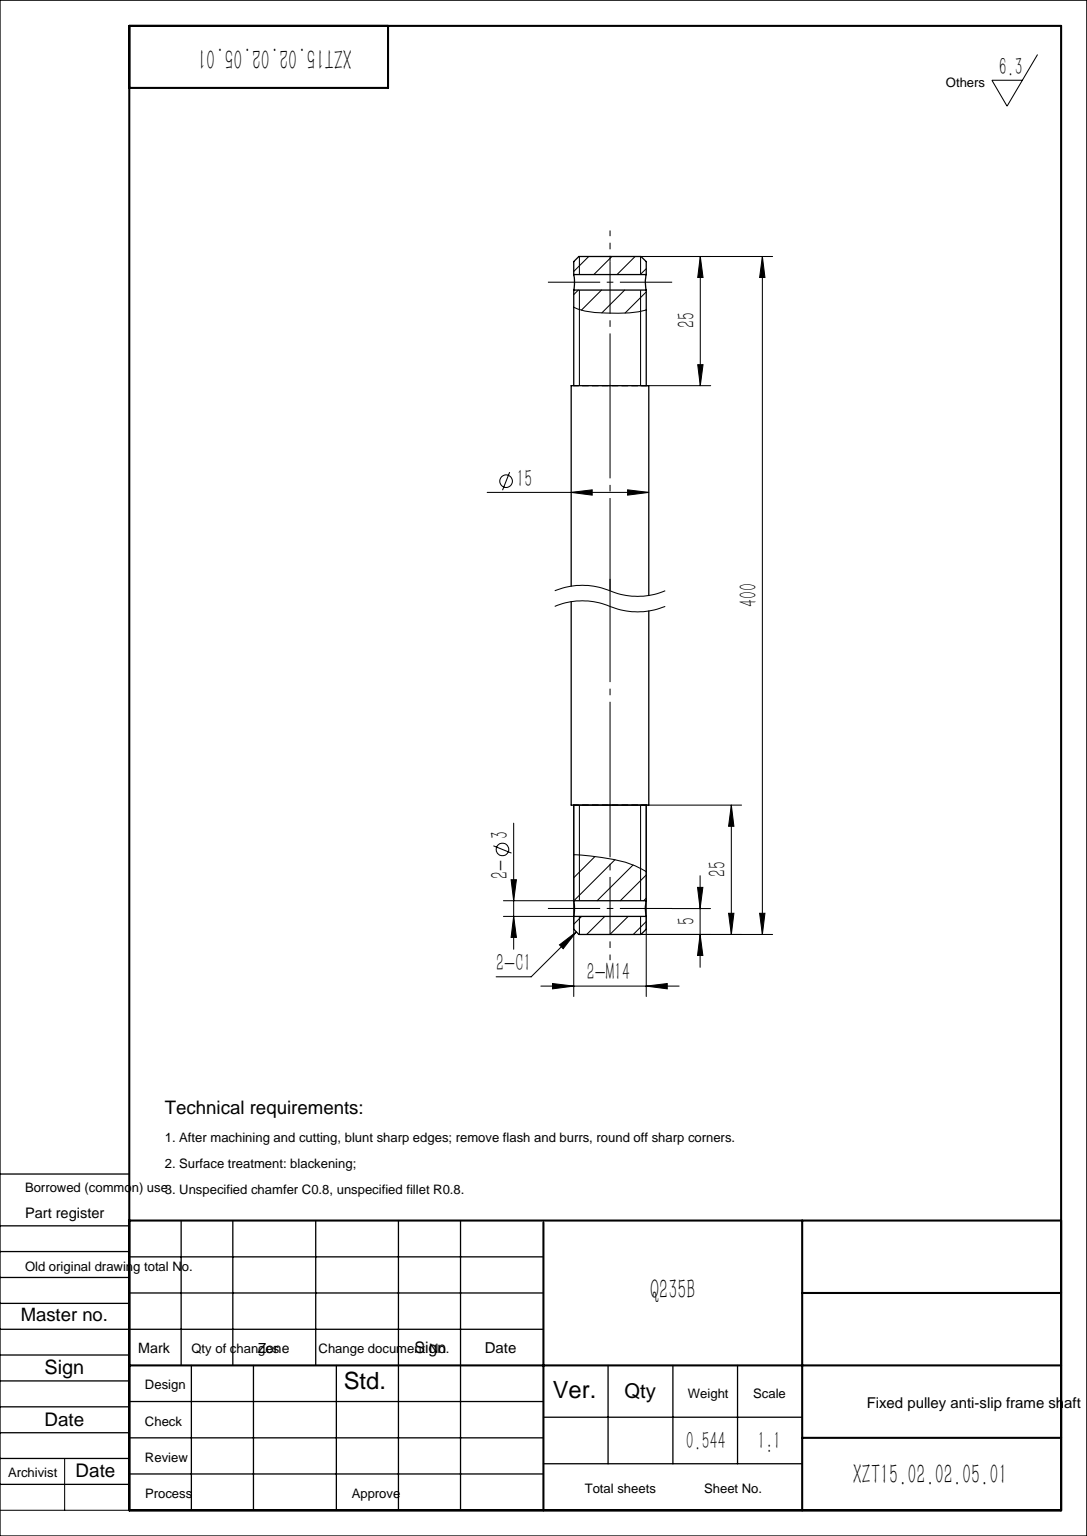
from build123d import *

# Parameters (mm, degrees)
CHAMFER1_SIZE           = 1
CUT_EXTRUDE1_DEPTH      = 401.140600289
CUT_EXTRUDE1_DEPTH_BACK = 401.140600289
SKETCH3_R               = 1.5


with BuildPart() as part:
    # Sketch1 → Revolve1 (revolve)
    with BuildSketch(Plane.XY, mode=Mode.PRIVATE) as revolve1_sk:
        Polygon((0, 0), (7, 0), (7, 25), (7.5, 25), (7.5, 375), (7, 375), (7, 400), (0, 400), align=None)
    revolve(revolve1_sk.sketch.rotate(Axis((0, 0, 0), (0, -1, 0)), 90), axis=Axis((0, 0, 0), (0, -1, 0)))

    # Chamfer1
    chamfer1_edges = [part.edges().sort_by_distance(p)[0] for p in [
        (0, 400, -7),
        (0, 0, -7),
    ]]
    chamfer(chamfer1_edges, length=CHAMFER1_SIZE)

    # Sketch3 → Cut-Extrude1 (cut, two sides: drawn at the far end of the back side and taken through both)
    with BuildSketch(Plane(origin=(0, 0, 0), x_dir=(0, 0, -1), z_dir=(1, 0, 0)).offset(-CUT_EXTRUDE1_DEPTH_BACK)):
        with Locations((0, 395)):
            Circle(SKETCH3_R)
        with Locations((0, 5)):
            Circle(SKETCH3_R)
    extrude(amount=CUT_EXTRUDE1_DEPTH + CUT_EXTRUDE1_DEPTH_BACK, mode=Mode.SUBTRACT)


solid = part.part
